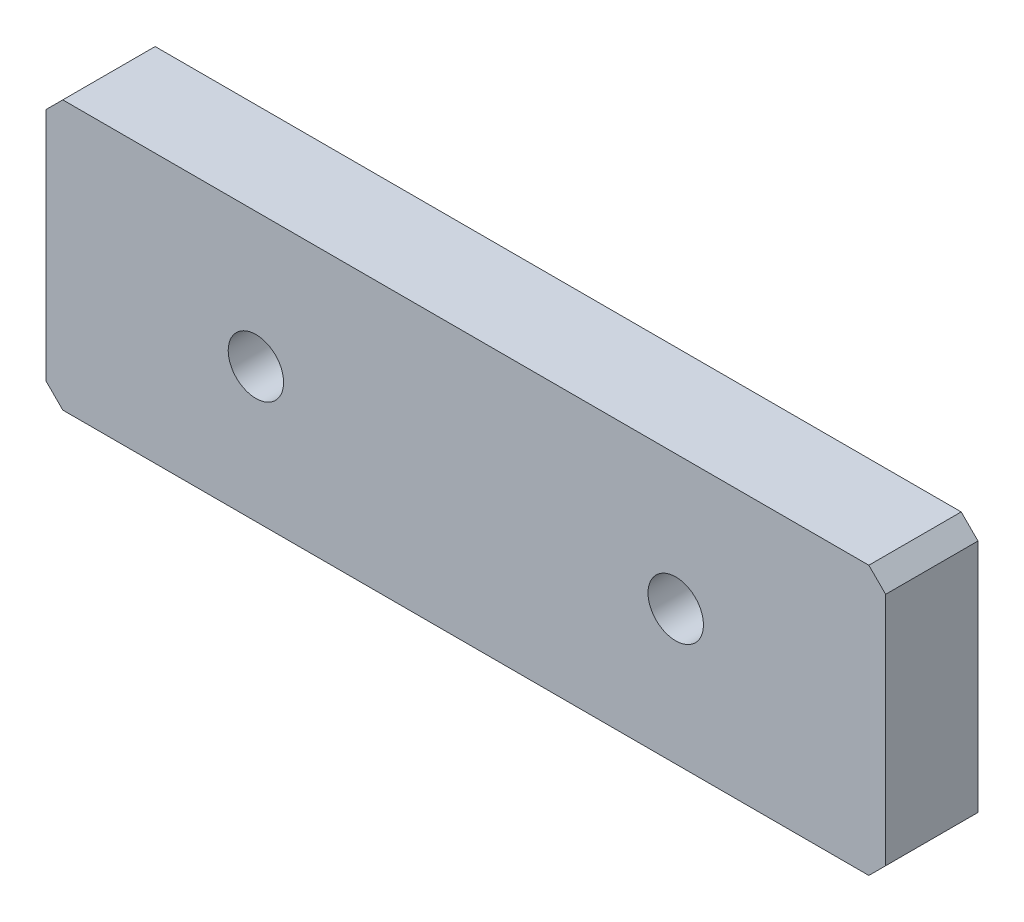
SolidWorks part; units mm, degrees
material "6061 合金"
ref_plane "前视基准面" through (0, 0, 0) normal (0, 0, 1) x (1, 0, 0)
ref_plane "上视基准面" through (0, 0, 0) normal (0, 1, 0) x (1, 0, 0)
ref_plane "右视基准面" through (0, 0, 0) normal (1, 0, 0) x (0, 0, -1)
sketch "草图1" plane through (0, 0, 0) normal (0, 0, 1) x (1, 0, 0)
  line L1 (-25, 8) -> (25, 8)
  line L2 (-25, 8) -> (-25, -8)
  line L3 (-25, -8) -> (25, -8)
  line L4 (25, 8) -> (25, -8)
  line L5 (-25, 8) -> (25, -8) construction
  line L6 (-25, -8) -> (25, 8) construction
  point P0 (0, 0)
  dimension "D1" = 16
  dimension "D2" = 50
extrude "凸台-拉伸1" add sketch "草图1" along normal mid plane 5.5
hole_wizard "M4 螺纹孔1" positions "草图3" profile "草图2" tap size "M4" standard "GB" end condition through all
sketch "草图3" plane through (0, 0, -2.75) normal (0, 0, -1) x (-1, 0, 0)
  point P0 (12.5, 0)
  point P2 (-12.5, 0)
  dimension "D1" = 12.5
sketch "草图2" plane through (-12.5, 0, -2.75) normal (1, 0, 0) x (0, 1, 0)
  line L0 (0, 0) -> (0, 5.5)
  line L1 (0, 5.5) -> (1.65, 5.5)
  line L2 (1.65, 5.5) -> (1.65, 0)
  line L5 (1.65, 0) -> (0, 0)
  line L11 (0, -6.35) -> (0, 107.95) construction
  dimension "通孔螺纹孔钻头直径" = 3.3
  dimension "通孔螺纹孔钻头深度" = 5.5
cosmetic thread "孔螺蚊线1" parameters "D2"=4
cosmetic thread "孔螺蚊线2" parameters "D2"=4
chamfer "倒角1" distance 1 angle 45 4 edges at (-25, -8, 0) (-25, 8, 0) (25, -8, 0) (25, 8, 0)
